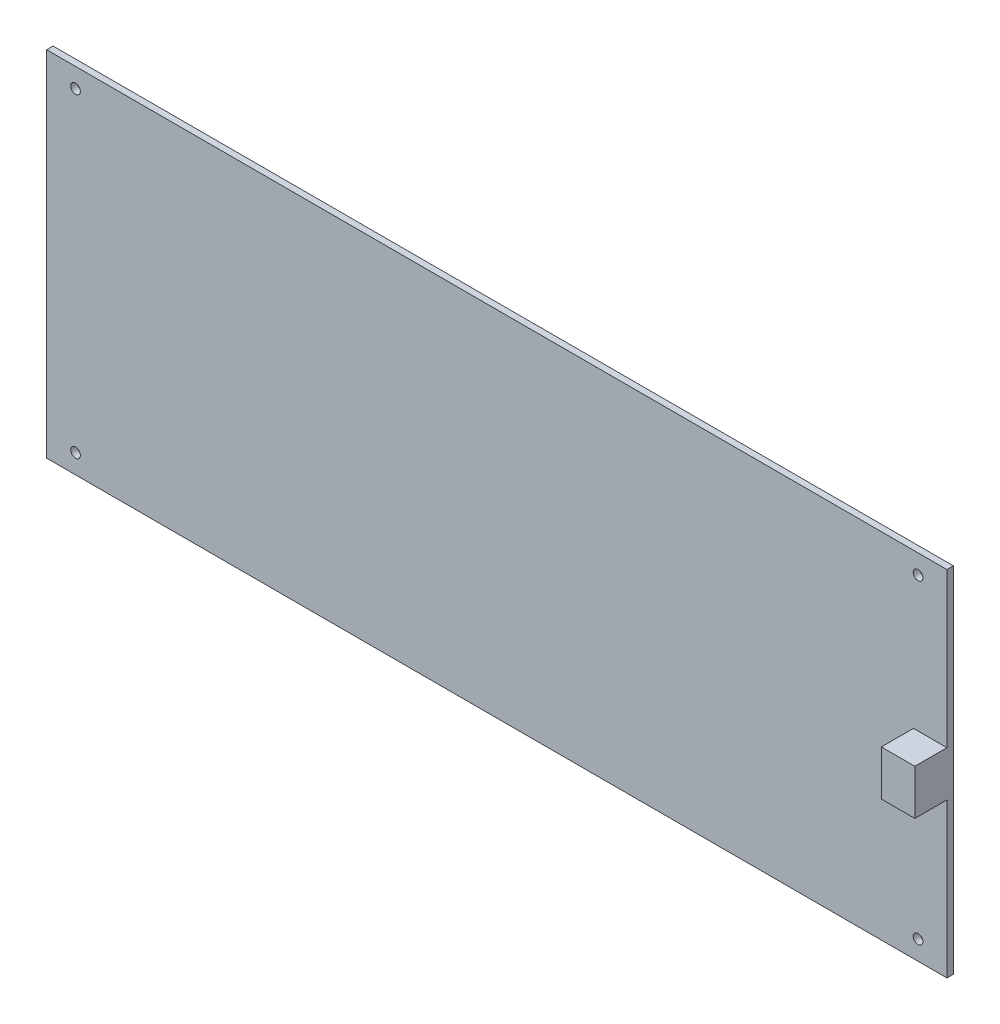
SolidWorks part; units mm, degrees
ref_plane "Front Plane" through (0, 0, 0) normal (0, 0, 1) x (1, 0, 0)
ref_plane "Top Plane" through (0, 0, 0) normal (0, 1, 0) x (1, 0, 0)
ref_plane "Right Plane" through (0, 0, 0) normal (1, 0, 0) x (0, 0, -1)
other "Configuration Table"
sketch "Sketch1" plane through (0, 0, 0) normal (0, 0, 1) x (1, 0, 0)
  line L1 (-70, 27.5) -> (70, 27.5)
  line L2 (-70, 27.5) -> (-70, -27.5)
  line L3 (-70, -27.5) -> (70, -27.5)
  line L4 (70, 27.5) -> (70, -27.5)
  line L5 (-70, 27.5) -> (70, -27.5) construction
  line L6 (-70, -27.5) -> (70, 27.5) construction
  line L7 (-65.5, 24.5) -> (65.5, 24.5) construction
  line L8 (-65.5, 24.5) -> (-65.5, -24.5) construction
  line L9 (-65.5, -24.5) -> (65.5, -24.5) construction
  line L10 (65.5, 24.5) -> (65.5, -24.5) construction
  line L11 (-65.5, 24.5) -> (65.5, -24.5) construction
  line L12 (-65.5, -24.5) -> (65.5, 24.5) construction
  circle A0 centre (-65.5, -24.5) radius 0.75
  circle A1 centre (-65.5, 24.5) radius 0.75
  circle A2 centre (65.5, 24.5) radius 0.75
  circle A3 centre (65.5, -24.5) radius 0.75
  point P0 (0, 0)
  point P6 (0, 0)
  dimension "D5" = 1.5
  dimension "D1" = 140
  dimension "D2" = 55
  dimension "D3" = 49
  dimension "D4" = 131
extrude "Boss-Extrude1" add sketch "Sketch1" along normal blind 1
sketch "Sketch2" plane through (0, 0, 1) normal (0, 0, 1) x (1, 0, 0)
  line L0 (70, -27.5) -> (70, 27.5) construction
  line L1 (64.7907, 3.5125) -> (70, 3.5125)
  line L2 (64.7907, 3.5125) -> (64.7907, -3.5125)
  line L3 (64.7907, -3.5125) -> (70, -3.5125)
  line L4 (70, 3.5125) -> (70, -3.5125)
  line L5 (64.7907, 3.5125) -> (70, -3.5125) construction
  line L6 (64.7907, -3.5125) -> (70, 3.5125) construction
  point P0 (67.3953, 0)
extrude "Boss-Extrude2" add sketch "Sketch2" along normal blind 5
